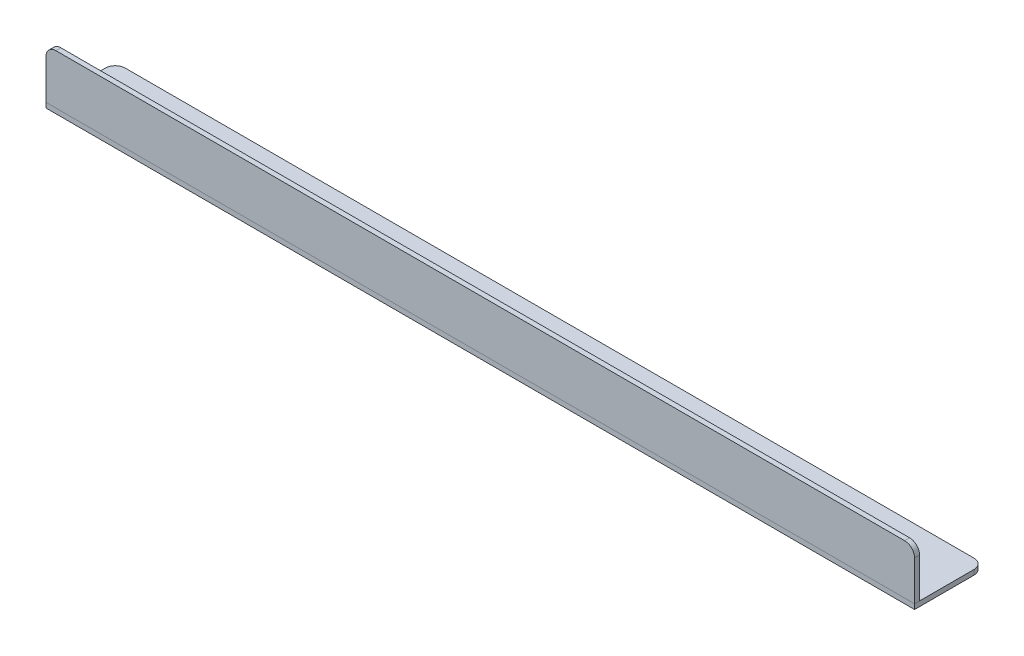
from build123d import *

# Parameters (mm, degrees)
SKETCH_1_W      = 1747.5
SKETCH_1_H      = 139.4
EXTRUDE_1_DEPTH = 10
SKETCH_2_W      = 1747.5
SKETCH_2_H      = 100
EXTRUDE_2_DEPTH = 10
EXTRUDE_3_DEPTH = 5
FILLET_1_R      = 20
FILLET_2_R      = 20


with BuildPart() as part:
    # 草图1 → 凸台-拉伸1 (new body)
    with BuildSketch(Plane(origin=(0, 0, 0), x_dir=(1, 0, 0), z_dir=(0, 1, 0))):
        Rectangle(SKETCH_1_W, SKETCH_1_H)
    extrude(amount=EXTRUDE_1_DEPTH)

    # 圆角2
    fillet_2_edges = [part.edges().sort_by_distance(p)[0] for p in [
        (-873.75, 5, -69.7),
        (873.75, 5, -69.7),
    ]]
    fillet(fillet_2_edges, radius=FILLET_2_R)


with BuildPart() as body_2:
    # 草图2 → 凸台-拉伸2 (new body)
    with BuildSketch(Plane.XY.offset(69.7)):
        with Locations((0, 60)):
            Rectangle(SKETCH_2_W, SKETCH_2_H)
    extrude(amount=-EXTRUDE_2_DEPTH)

    # 圆角1
    fillet_1_edges = [body_2.edges().sort_by_distance(p)[0] for p in [
        (-873.75, 110, 64.7),
        (873.75, 110, 64.7),
    ]]
    fillet(fillet_1_edges, radius=FILLET_1_R)


with BuildPart() as body_3:
    # 草图3 → 凸台-拉伸3 (new, symmetric)
    with BuildSketch(Plane(origin=(0, 0, 0), x_dir=(0, 0, -1), z_dir=(1, 0, 0))):
        Polygon((0, 10), (-59.7, 60), (-59.7, 10), align=None)
    extrude(amount=EXTRUDE_3_DEPTH, both=True)


solid = Compound([part.part, body_2.part, body_3.part])
